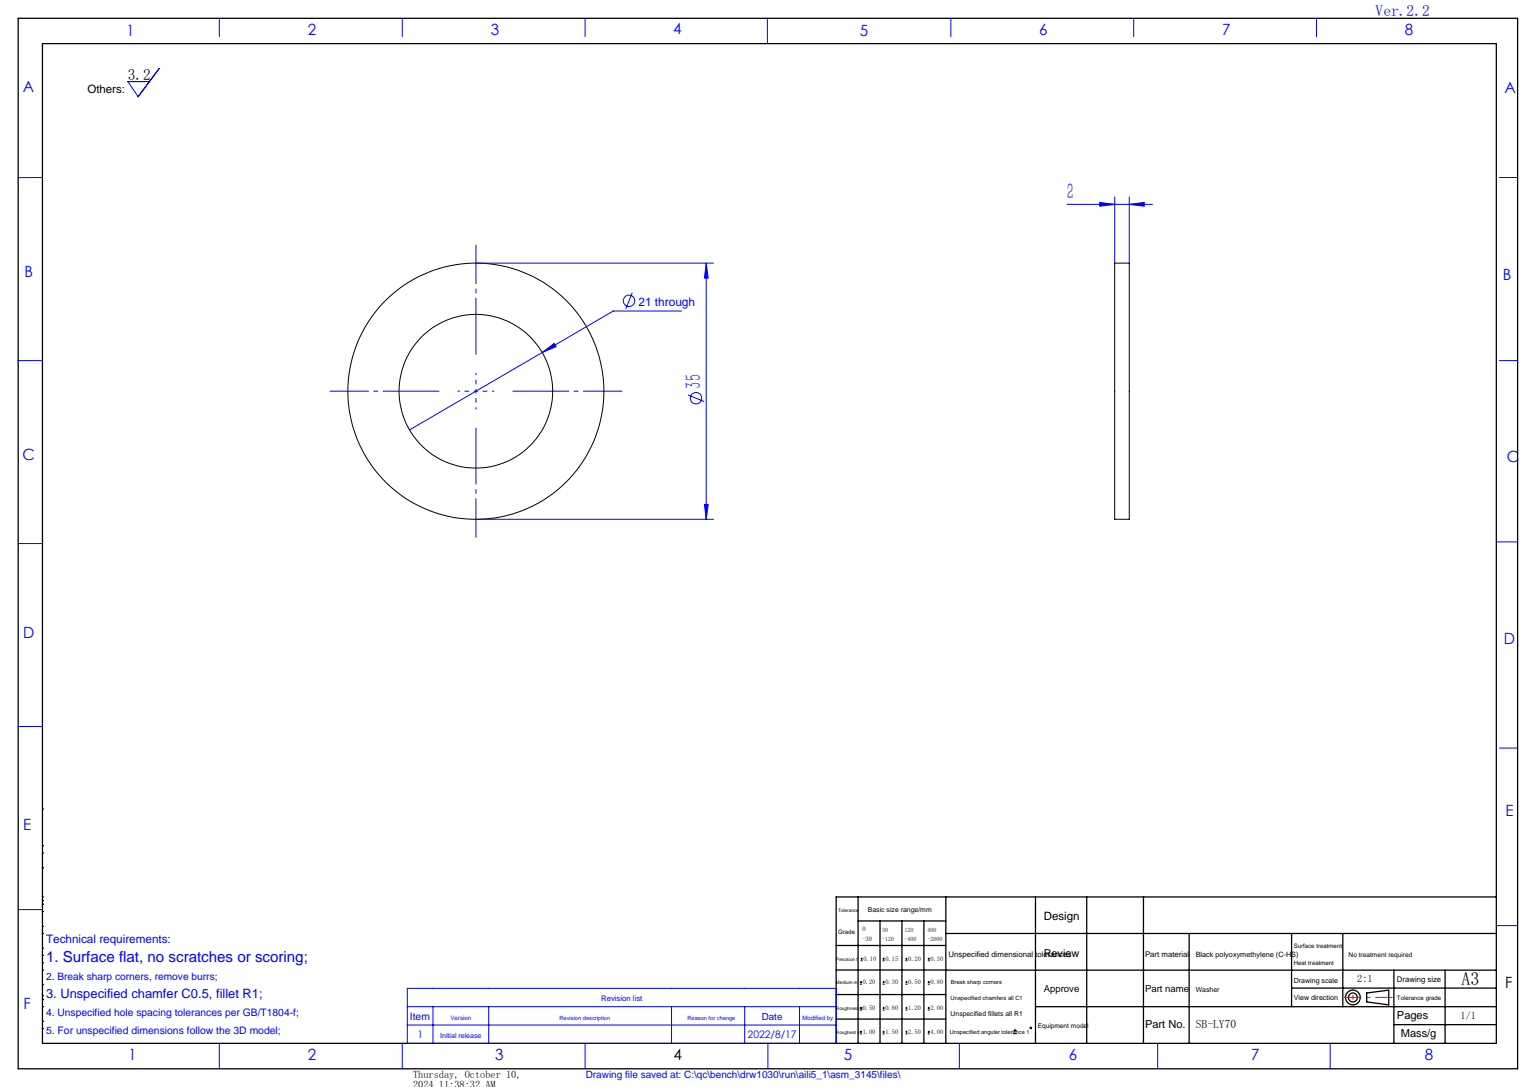
SolidWorks part; units mm, degrees
material "黑色赛钢(C-HS)"
ref_plane "前视基准面" through (0, 0, 0) normal (0, 0, 1) x (1, 0, 0)
ref_plane "上视基准面" through (0, 0, 0) normal (0, 1, 0) x (1, 0, 0)
ref_plane "右视基准面" through (0, 0, 0) normal (1, 0, 0) x (0, 0, -1)
sketch "草图1" plane through (0, 0, 0) normal (0, 0, 1) x (1, 0, 0)
  circle A0 centre (0, 0) radius 17.5
  circle A1 centre (0, 0) radius 10.5
  dimension "D1" = 35
  dimension "D2" = 21
extrude "凸台-拉伸1" add sketch "草图1" along normal blind 2
